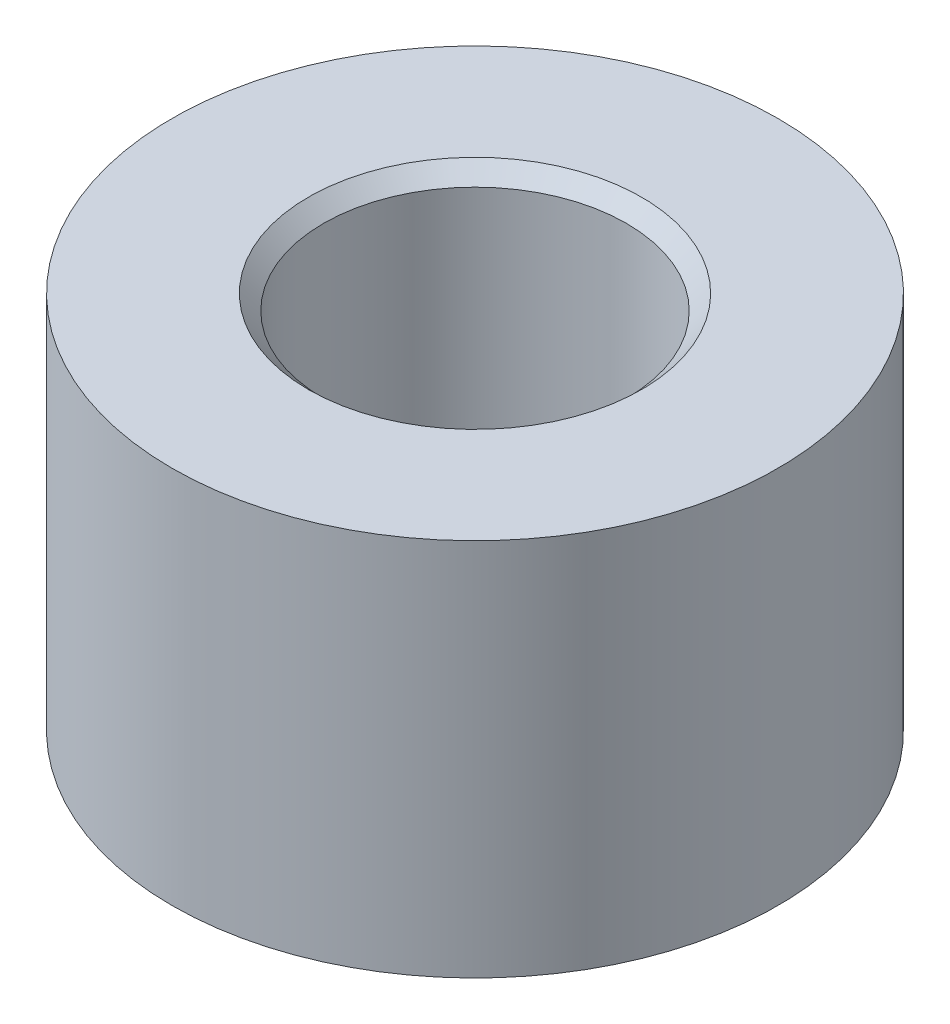
from build123d import *

# Parameters (mm, degrees)
SKETCH_1_R          = 2
SKETCH_1_R_2        = 1
EXTRUDE_1_DEPTH     = 2.5
CHAMFER_C0_1_1_SIZE = 0.1


with BuildPart() as part:
    # 草图1 → 凸台-拉伸1 (new body)
    with BuildSketch(Plane(origin=(0, 0, 0), x_dir=(1, 0, 0), z_dir=(0, 1, 0))):
        with Locations(Location((0, 0, 0), (0, 0, 270))):
            Circle(SKETCH_1_R)
        with Locations(Location((0, 0, 0), (0, 0, 270))):
            Circle(SKETCH_1_R_2, mode=Mode.SUBTRACT)
    extrude(amount=EXTRUDE_1_DEPTH)

    # C0.1 倒角1
    chamfer_c0_1_1_edges = [part.edges().sort_by_distance(p)[0] for p in [
        (0, 0, -1),
        (0, 2.5, -1),
    ]]
    chamfer(chamfer_c0_1_1_edges, length=CHAMFER_C0_1_1_SIZE)


solid = part.part
